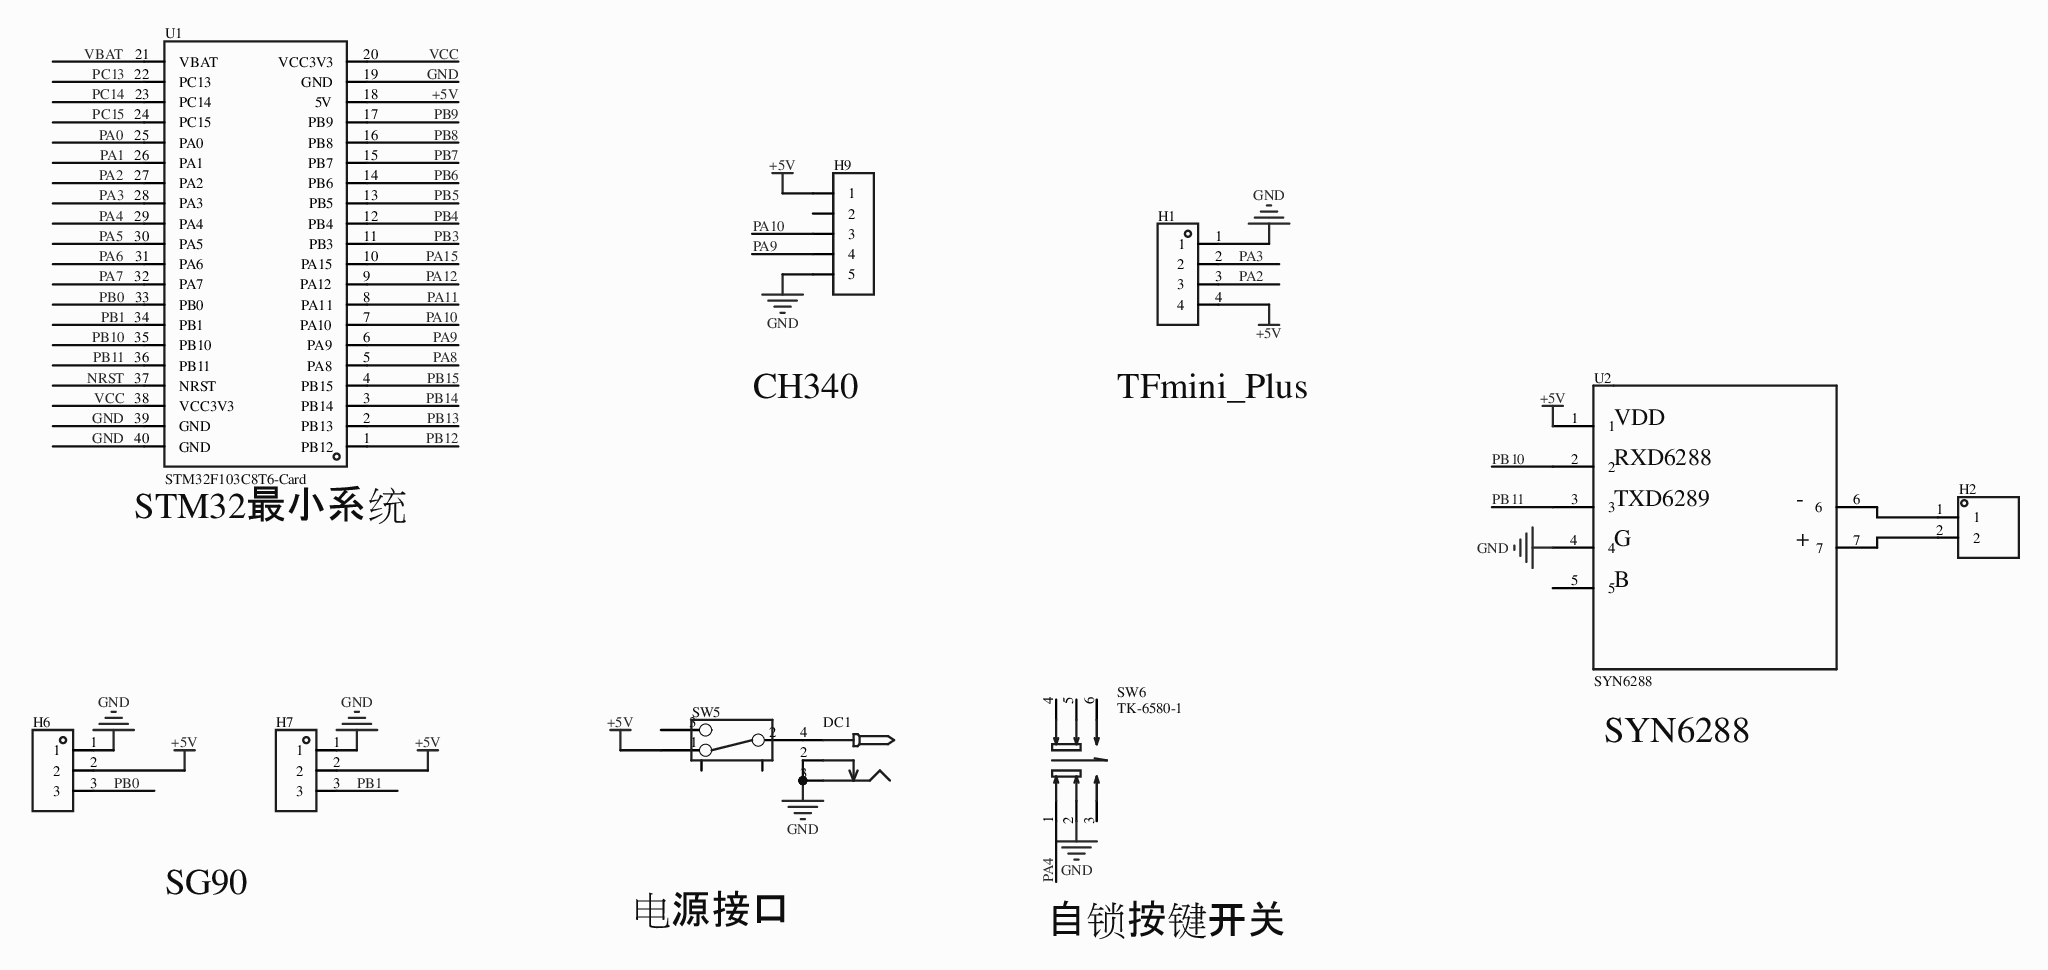
[diagram p0: MISC51113-3.schdoc]
# Altium project MISC51113-2.PrjPcb
1 sheet, 10 parts. Net scope: global (net labels, ports and power ports of the same name join across sheets).
Board file: MISC51113.pcbdoc

## Sheet MISC51113-3.schdoc
size 297 x 209 mm; Version: V1.0; @Project Name: MISC51113; @Page Count: 1; @Update Date: 2026-05-22; @Create Date: 2026-05-22; @Schematic Name: MISC51113; @Page No: 1; @Create Time: 23:22:16; @Update Time: 17:32:40; @Board Name: MISC51113

### Parts
DC1  (no value)  [DC-2.0]
H1  (no value)  [HDR-TH_4P-P2.54-V-F]
H2  (no value)  [HDR-TH_2P-P2.54-V-M-1]
H6  (no value)  [HDR-TH_3P-P2.54-V-F]
H7  (no value)  [HDR-TH_3P-P2.54-V-F]
H9  (no value)  [HDR-TH_5P-P2.54-V-F]
SW5  (no value)  [拨动开关]
SW6  TK-6580-1  [SW-TH_TK-6580-1]
U1  STM32F103C8T6-Card  [CONN-TH_L53.3-W22.9_STM32F103C8T6-CARD]
U2  SYN6288  [SYN6288]

### Nets
+5V: H1.4 H6.2 H7.2 H9.1 SW5.1 U1.18(5V) U2.1
GND: DC1.2 DC1.3 H1.1 H6.1 H7.1 H9.5 SW6.2 U1.19(GND) U1.39(GND) U1.40(GND) U2.4
NRST: U1.37(NRST)
PA0: U1.25(PA0)
PA1: U1.26(PA1)
PA2: H1.3 U1.27(PA2)
PA3: H1.2 U1.28(PA3)
PA4: SW6.1 U1.29(PA4)
PA5: U1.30(PA5)
PA6: U1.31(PA6)
PA7: U1.32(PA7)
PA8: U1.5(PA8)
PA9: H9.4 U1.6(PA9)
PA10: H9.3 U1.7(PA10)
PA11: U1.8(PA11)
PA12: U1.9(PA12)
PA15: U1.10(PA15)
PB0: H6.3 U1.33(PB0)
PB1: H7.3 U1.34(PB1)
PB3: U1.11(PB3)
PB4: U1.12(PB4)
PB5: U1.13(PB5)
PB6: U1.14(PB6)
PB7: U1.15(PB7)
PB8: U1.16(PB8)
PB9: U1.17(PB9)
PB10: U1.35(PB10) U2.2
PB11: U1.36(PB11) U2.3
PB12: U1.1(PB12)
PB13: U1.2(PB13)
PB14: U1.3(PB14)
PB15: U1.4(PB15)
PC13: U1.22(PC13)
PC14: U1.23(PC14)
PC15: U1.24(PC15)
VBAT: U1.21(VBAT)
VCC: U1.20(VCC3V3) U1.38(VCC3V3)
NetDC1_4: DC1.4 SW5.2
NetH2_1: H2.1 U2.6
NetH2_2: H2.2 U2.7

Not connected (* = marked no-connect by the designer): H9 2; SW5 3 4 5; SW6 3 4 5 6; U2 5

### Notes on the sheet
- CH340
- (near H1) TFmini_Plus
- (near U1) STM32最小系统
- SYN6288
- SG90
- 电源接口
- 自锁按键开关

### Library data of the parts
DC1 = DC-005_2.0: Symbol: DC电源接口; ConvertToPcb: yes; ModelId: f5f20b8a2308479b936ba3c2698865bb0819f05c4eef4c71ace90d822a990e87; ModelName: DC-IN-TH_DC-5520-1; ModelTransform: 372.05,551.18,582.68,90,0,0,137.8,0,-149.61; Device: DC-005_2.0; AddInBom: yes; Supplier Footprint: 插件; FootprintName: DC-2.0
H1 = HDR-F_2.54_1x4P: Symbol: 2.54-1*4P母; ConvertToPcb: yes; ModelId: d187812051054f85879fcaa51a310d8e0819f05c4eef4c71ace90d822a990e87; ModelTransform: 419.6842,98.464,0,0,0,0,0,0,-118.11; Device: HDR-F_2.54_1x4P; AddInBom: yes; SupplierPart: C2718488; Supplier Footprint: 插件; FootprintName: HDR-TH_4P-P2.54-V-F; ModelName: HDR-TH_4P-P2.54-V-F
H2 = HDR-M_2.54_1x2P: Symbol: 210S-1*2P L=11.6MMGold-plated black; ConvertToPcb: yes; ModelId: 79b2e9f2d70a4d68a1b7098f27c6d4c50819f05c4eef4c71ace90d822a990e87; ModelName: HDR-M-2.54_1x2; ModelTransform: 200,100,0,0,0,0,0,0,-118.11; Device: HDR-M_2.54_1x2P; AddInBom: yes; SupplierPart: C124375; Supplier Footprint: 插件; FootprintName: HDR-TH_2P-P2.54-V-M-1
H6 H7 = HDR-F_2.54_1x3P: Symbol: PM254V-11-03-H85; ConvertToPcb: yes; ModelId: f3b3cc5aae9641bf9e56fc160cef875b; ModelName: HDR2.54-F-LI-1X3P; ModelTransform: 299.9994,100,0,0,0,0,0,0,-118.11; Device: HDR-F_2.54_1x3P; FootprintName: HDR-TH_3P-P2.54-V-F; AddInBom: yes; SupplierPart: C541850; Supplier Footprint: 插件
H9 = HDR-F_2.54_1x5P: Symbol: Header-Female-2.54_1x5; 3D Model: f49cb6116a3d45e5a64915bf3e00773f; 3D Model Transform: 519.684,98.464,0,0,0,0,0,0,-124.016; ConvertToPcb: yes; Device: HDR-F_2.54_1x5P; Supplier Part: C50950; Supplier Footprint: 插件; AddInBom: yes; FootprintName: HDR-TH_5P-P2.54-V-F; ModelName: HDR-TH_5P-P2.54-V-F
SW5 = 拨动开关_正: ConvertToPcb: yes; ModelId: 4321fe59a4074cbfb4989553f297c68f0819f05c4eef4c71ace90d822a990e87; ModelName: SW-TH_SS-12D02-VG4; ModelTransform: 370.09,208.7,472.35,0,0,0,0,0,-110; Device: 拨动开关_正; Symbol: 拨动开关; FootprintName: 拨动开关; AddInBom: yes; Supplier Footprint: 插件
SW6 = TK-6580-1: Manufacturer: Yuandi(元迪); AddInBom: yes; ModelId: e510c342420842aebf6eaf4acf4e9fda0819f05c4eef4c71ace90d822a990e87; ModelTransform: 228.3460083128025,228.3460083128025,533.4635,0,0,0,0,0,-137.79528; Symbol: TK-6580-1; Device: TK-6580-1; ConvertToPcb: yes; Supplier: LCSC; SupplierPart: C528778; ManufacturerPart: TK-6580-1; JLCPCB Part Class: Extended Part; FootprintName: SW-TH_TK-6580-1; ModelName: SW-TH_TK-6580-1
U1 = STM32F103C8T6-Card: AddInBom: yes; Device: STM32F103C8T6-Card; Symbol: STM32F103C8T6-CARD; FootprintName: CONN-TH_L53.3-W22.9_STM32F103C8T6-CARD; LCSC Part Name: STM32F103C8T6-Card; SupplierPart: C9900077949; ManufacturerPart: STM32F103C8T6-Card; Supplier Footprint: 插件; Supplier: LCSC; ConvertToPcb: yes
U2 = SYN6288: AddInBom: yes; Symbol: SYN6288; Device: SYN6288; FootprintName: SYN6288; ConvertToPcb: yes